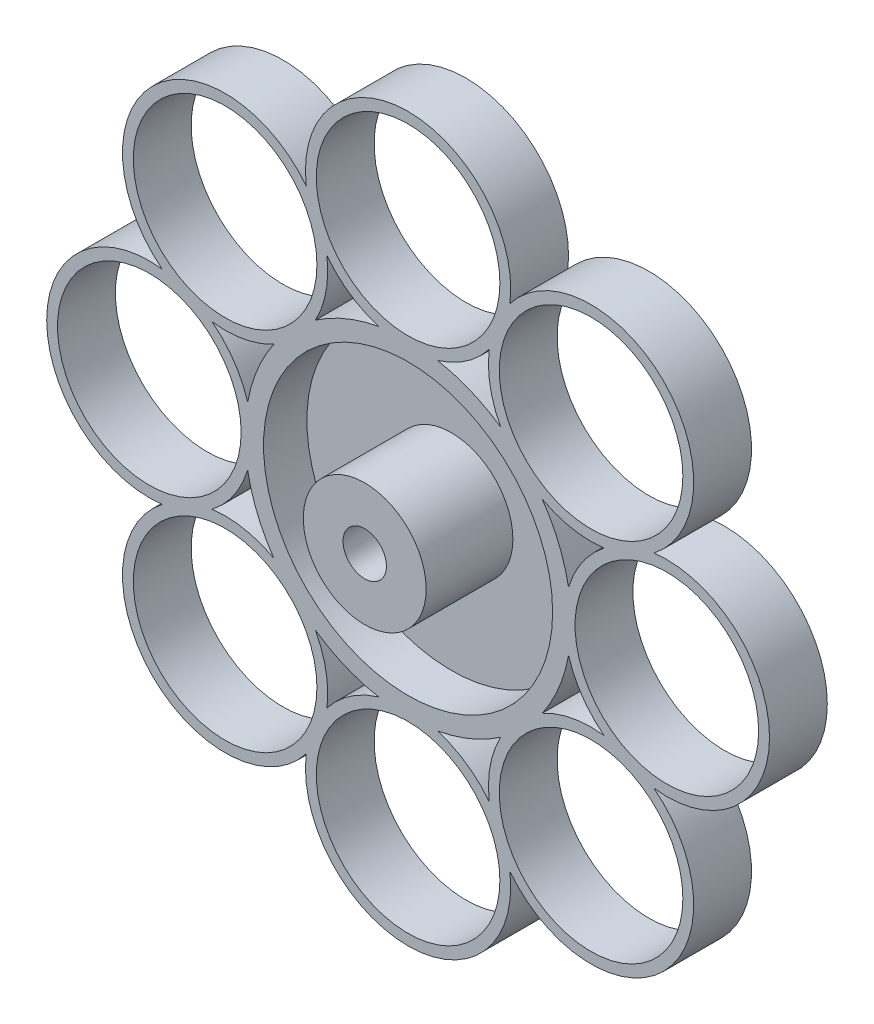
from build123d import *

# Parameters (mm, degrees)
SKETCH1_R           = 3
SKETCH1_R_2         = 12.7
BOSS_EXTRUDE1_DEPTH = 8
SKETCH4_R           = 20
SKETCH4_R_2         = 8.5
CUT_EXTRUDE2_DEPTH  = 6
SKETCH5_R           = 8.5
SKETCH5_R_2         = 3
BOSS_EXTRUDE3_DEPTH = 6


with BuildPart() as part:
    # Sketch1 → Boss-Extrude1 (new body)
    with BuildSketch(Plane.XY):
        with BuildLine():
            ThreePointArc((-14.086428596, 34.007646961), (-35.355339059, 35.355339059), (-34.007646961, 14.086428596))
            ThreePointArc((-34.007646961, 14.086428596), (-50, 0), (-34.007646961, -14.086428596))
            ThreePointArc((-34.007646961, -14.086428596), (-35.355339059, -35.355339059), (-14.086428596, -34.007646961))
            ThreePointArc((-14.086428596, -34.007646961), (0, -50), (14.086428596, -34.007646961))
            ThreePointArc((14.086428596, -34.007646961), (35.355339059, -35.355339059), (34.007646961, -14.086428596))
            ThreePointArc((34.007646961, -14.086428596), (50, 0), (34.007646961, 14.086428596))
            ThreePointArc((34.007646961, 14.086428596), (35.355339059, 35.355339059), (14.086428596, 34.007646961))
            ThreePointArc((14.086428596, 34.007646961), (0, 50), (-14.086428596, 34.007646961))
        make_face()
        Circle(SKETCH1_R, mode=Mode.SUBTRACT)
        with Locations((0, 35.8)):
            Circle(SKETCH1_R_2, mode=Mode.SUBTRACT)
        with Locations((25.314422766, 25.314422766)):
            Circle(SKETCH1_R_2, mode=Mode.SUBTRACT)
        with Locations((35.8, 0)):
            Circle(SKETCH1_R_2, mode=Mode.SUBTRACT)
        with Locations((25.314422766, -25.314422766)):
            Circle(SKETCH1_R_2, mode=Mode.SUBTRACT)
        with Locations((0, -35.8)):
            Circle(SKETCH1_R_2, mode=Mode.SUBTRACT)
        with Locations((-25.314422766, -25.314422766)):
            Circle(SKETCH1_R_2, mode=Mode.SUBTRACT)
        with Locations((-35.8, 0)):
            Circle(SKETCH1_R_2, mode=Mode.SUBTRACT)
        with Locations((-25.314422766, 25.314422766)):
            Circle(SKETCH1_R_2, mode=Mode.SUBTRACT)
        with BuildLine():
            ThreePointArc((-11.227994171, 27.106775805), (-8.03692429, 24.093256305), (-4.078024952, 22.198172458))
            ThreePointArc((-4.078024952, 22.198172458), (-8.637031526, 20.85163865), (-12.812879177, 18.580077372))
            ThreePointArc((-12.812879177, 18.580077372), (-11.353541248, 22.719468579), (-11.227994171, 27.106775805))
        make_face(mode=Mode.SUBTRACT)
        with BuildLine():
            ThreePointArc((11.227994171, 27.106775805), (11.353541248, 22.719468579), (12.812879177, 18.580077372))
            ThreePointArc((12.812879177, 18.580077372), (8.637031526, 20.85163865), (4.078024952, 22.198172458))
            ThreePointArc((4.078024952, 22.198172458), (8.03692429, 24.093256305), (11.227994171, 27.106775805))
        make_face(mode=Mode.SUBTRACT)
        with BuildLine():
            ThreePointArc((27.106775805, 11.227994171), (24.093256305, 8.03692429), (22.198172458, 4.078024952))
            ThreePointArc((22.198172458, 4.078024952), (20.85163865, 8.637031526), (18.580077372, 12.812879177))
            ThreePointArc((18.580077372, 12.812879177), (22.719468579, 11.353541248), (27.106775805, 11.227994171))
        make_face(mode=Mode.SUBTRACT)
        with BuildLine():
            ThreePointArc((27.106775805, -11.227994171), (22.719468579, -11.353541248), (18.580077372, -12.812879177))
            ThreePointArc((18.580077372, -12.812879177), (20.85163865, -8.637031526), (22.198172458, -4.078024952))
            ThreePointArc((22.198172458, -4.078024952), (24.093256305, -8.03692429), (27.106775805, -11.227994171))
        make_face(mode=Mode.SUBTRACT)
        with BuildLine():
            ThreePointArc((11.227994171, -27.106775805), (8.03692429, -24.093256305), (4.078024952, -22.198172458))
            ThreePointArc((4.078024952, -22.198172458), (8.637031526, -20.85163865), (12.812879177, -18.580077372))
            ThreePointArc((12.812879177, -18.580077372), (11.353541248, -22.719468579), (11.227994171, -27.106775805))
        make_face(mode=Mode.SUBTRACT)
        with BuildLine():
            ThreePointArc((-11.227994171, -27.106775805), (-11.353541248, -22.719468579), (-12.812879177, -18.580077372))
            ThreePointArc((-12.812879177, -18.580077372), (-8.637031526, -20.85163865), (-4.078024952, -22.198172458))
            ThreePointArc((-4.078024952, -22.198172458), (-8.03692429, -24.093256305), (-11.227994171, -27.106775805))
        make_face(mode=Mode.SUBTRACT)
        with BuildLine():
            ThreePointArc((-27.106775805, -11.227994171), (-24.093256305, -8.03692429), (-22.198172458, -4.078024952))
            ThreePointArc((-22.198172458, -4.078024952), (-20.85163865, -8.637031526), (-18.580077372, -12.812879177))
            ThreePointArc((-18.580077372, -12.812879177), (-22.719468579, -11.353541248), (-27.106775805, -11.227994171))
        make_face(mode=Mode.SUBTRACT)
        with BuildLine():
            ThreePointArc((-18.580077372, 12.812879177), (-20.85163865, 8.637031526), (-22.198172458, 4.078024952))
            ThreePointArc((-22.198172458, 4.078024952), (-24.093256305, 8.03692429), (-27.106775805, 11.227994171))
            ThreePointArc((-27.106775805, 11.227994171), (-22.719468579, 11.353541248), (-18.580077372, 12.812879177))
        make_face(mode=Mode.SUBTRACT)
    extrude(amount=BOSS_EXTRUDE1_DEPTH)

    # Sketch4 → Cut-Extrude2 (cut)
    with BuildSketch(Plane.XY.offset(8)):
        Circle(SKETCH4_R)
        Circle(SKETCH4_R_2, mode=Mode.SUBTRACT)
    extrude(amount=-CUT_EXTRUDE2_DEPTH, mode=Mode.SUBTRACT)

    # Sketch5 → Boss-Extrude3 (add)
    with BuildSketch(Plane.XY.offset(8)):
        Circle(SKETCH5_R)
        Circle(SKETCH5_R_2, mode=Mode.SUBTRACT)
    extrude(amount=BOSS_EXTRUDE3_DEPTH)


solid = part.part
